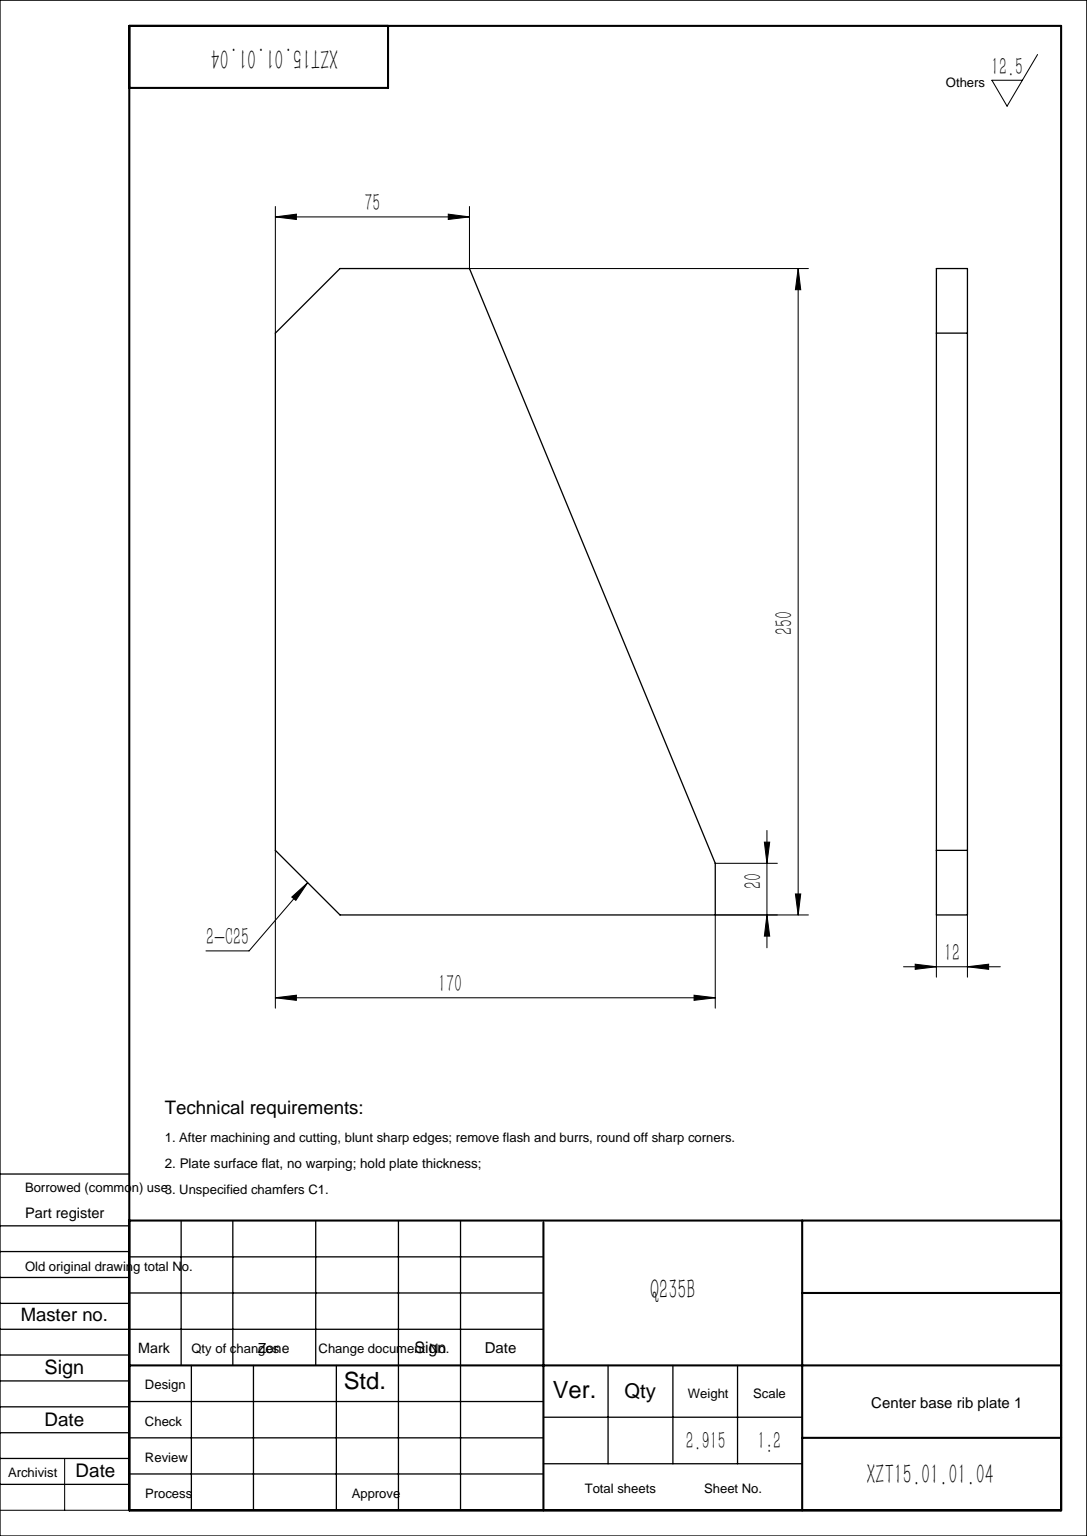
from build123d import *

# Parameters (mm, degrees)
BOSS_EXTRUDE1_DEPTH = 6
CHAMFER1_SIZE       = 25


with BuildPart() as part:
    # Sketch1 → Boss-Extrude1 (new, symmetric)
    with BuildSketch(Plane.XY):
        Polygon((0, 0), (170, 0), (170, 20), (75, 250), (0, 250), align=None)
    extrude(amount=BOSS_EXTRUDE1_DEPTH, both=True)

    # Chamfer1
    chamfer1_edges = [part.edges().sort_by_distance(p)[0] for p in [
        (0, 250, 0),
        (0, 0, 0),
    ]]
    chamfer(chamfer1_edges, length=CHAMFER1_SIZE)


solid = part.part
